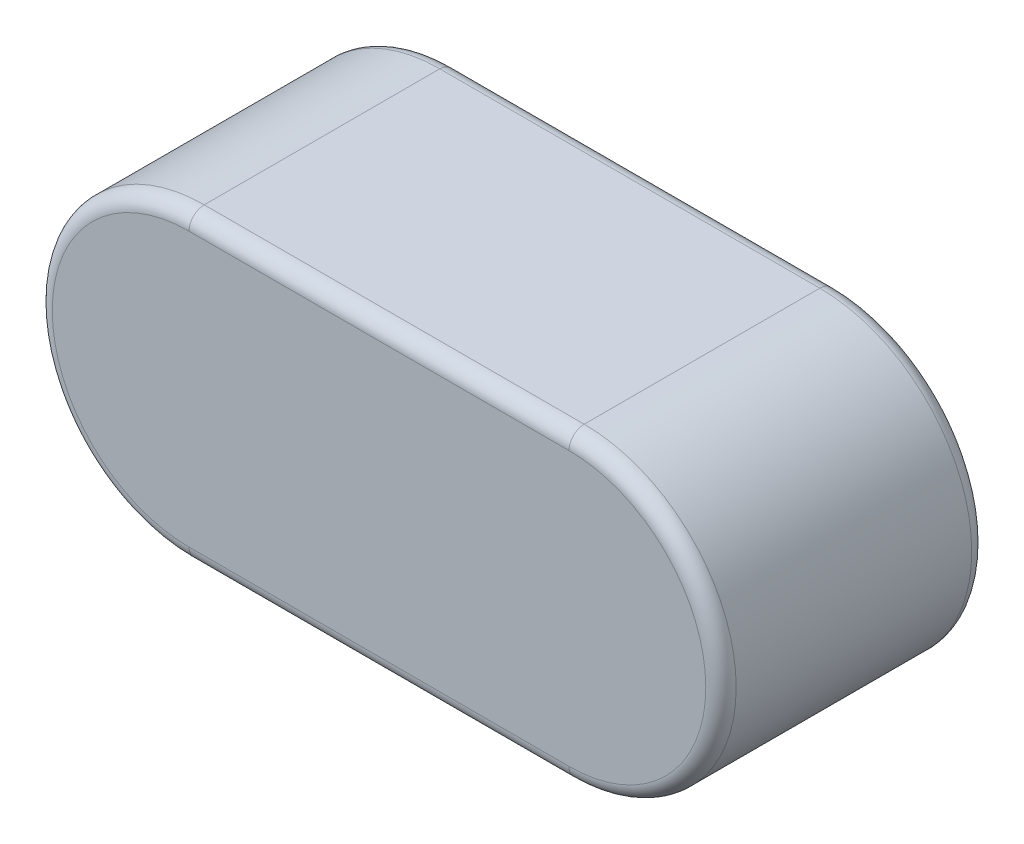
SolidWorks part; units mm, degrees
material "45"
ref_plane "基准面1" through (0, 0, 0) normal (0, 0, 1) x (1, 0, 0)
ref_plane "基准面2" through (0, 0, 0) normal (0, 1, 0) x (1, 0, 0)
ref_plane "基准面3" through (0, 0, 0) normal (1, 0, 0) x (0, 0, -1)
sketch "尺寸草图" plane through (0, 0, 0) normal (0, 0, 1) x (1, 0, 0)
  line L0 (-9, 0) -> (9, 0) construction
  point P3 (-7, 0)
  point P4 (-0.4, 0)
  point P5 (0, 0)
  point P8 (-8, 0)
  point P11 (0, 0)
sketch "草图1" plane through (0, 0, 0) normal (0, 0, 1) x (1, 0, 0)
  line L0 (-28.0599, 0) -> (30.562, 0) construction
  line L1 (-5, 4) -> (5, 4)
  line L2 (-5, -4) -> (5, -4)
  line L3 (0, 2.9108) -> (0, -2.1805) construction
  arc A0 (-5, 4) -> (-5, -4) centre (-5, 0) ccw
  arc A1 (5, 4) -> (5, -4) centre (5, 0) cw
extrude "基体-拉伸" add sketch "草图1" along normal blind 7
fillet "圆角1" radius 0.4 8 edges at (9, 0, 7) (0, 4, 7) (-9, 0, 7) (0, 4, 0) (9, 0, 0) (0, -4, 0) (-9, 0, 0) (0, -4, 7)
equation "\"D3@草图1\" = \"L@尺寸草图\""
equation "\"D1@草图1\" = \"b@尺寸草图\" / 2"
equation "\"D1@圆角1\" = \"r@尺寸草图\""
equation "\"D1@基体-拉伸\" = \"h@尺寸草图\""
